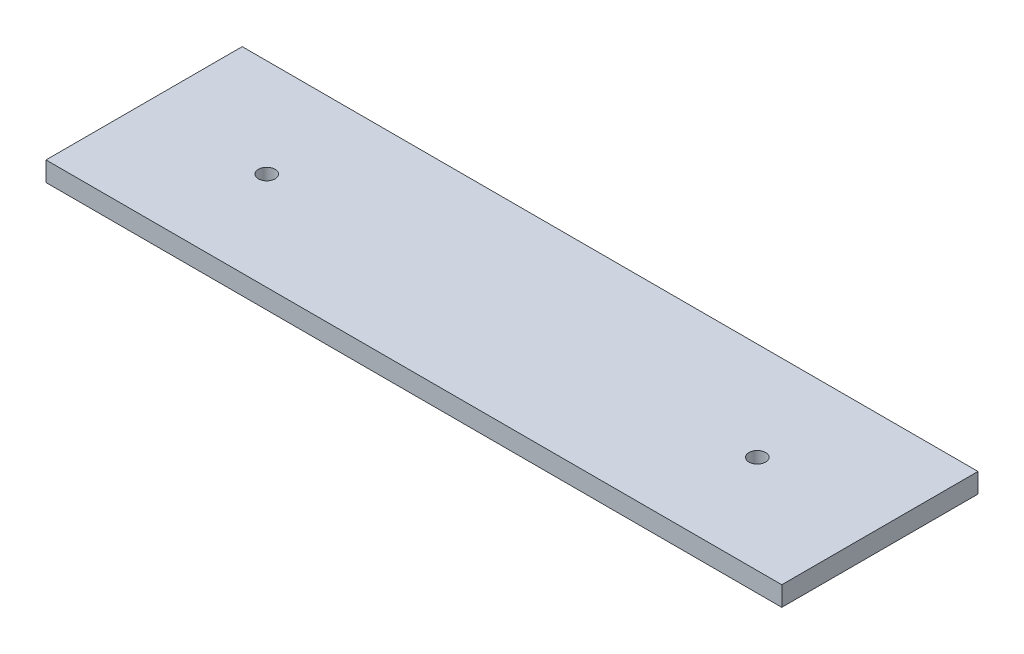
SolidWorks part; units mm, degrees
material "Q235"
ref_plane "Front" through (0, 0, 0) normal (0, 0, 1) x (1, 0, 0)
ref_plane "Top" through (0, 0, 0) normal (0, 1, 0) x (1, 0, 0)
ref_plane "Right" through (0, 0, 0) normal (1, 0, 0) x (0, 0, -1)
sketch "Sketch1" plane through (0, 0, 0) normal (0, 1, 0) x (1, 0, 0)
  line L1 (0, 0) -> (300, 0)
  line L2 (0, 0) -> (0, 80)
  line L3 (0, 80) -> (300, 80)
  line L4 (300, 0) -> (300, 80)
  dimension "D1" = 300
  dimension "D2" = 80
extrude "Boss-Extrude1" add sketch "Sketch1" along normal blind 8
hole_wizard "M8 Tapped Hole1" positions "Sketch3" profile "Sketch4" tap size "M8" standard "GB" end condition through all
sketch "Sketch3" plane through (0, 8, 0) normal (0, 1, 0) x (1, 0, 0)
  line L0 (150, 80) -> (150, 29.5912) construction
  line L1 (300, 80) -> (0, 80) construction
  point P0 (50, 40)
  point P2 (250, 40)
  dimension "D1" = 200
  dimension "D2" = 40
sketch "Sketch4" plane through (50, 8, -40) normal (1, 0, 0) x (0, 0, 1)
  line L0 (0, 0) -> (0, 8)
  line L1 (0, 8) -> (3.4, 8)
  line L2 (3.4, 8) -> (3.4, 0)
  line L5 (3.4, 0) -> (0, 0)
  line L11 (0, -6.35) -> (0, 107.95) construction
  dimension "通孔螺纹孔钻头直径" = 6.8
  dimension "通孔螺纹孔钻头深度" = 8
cosmetic thread "Hole thread1"
cosmetic thread "Hole thread2"
